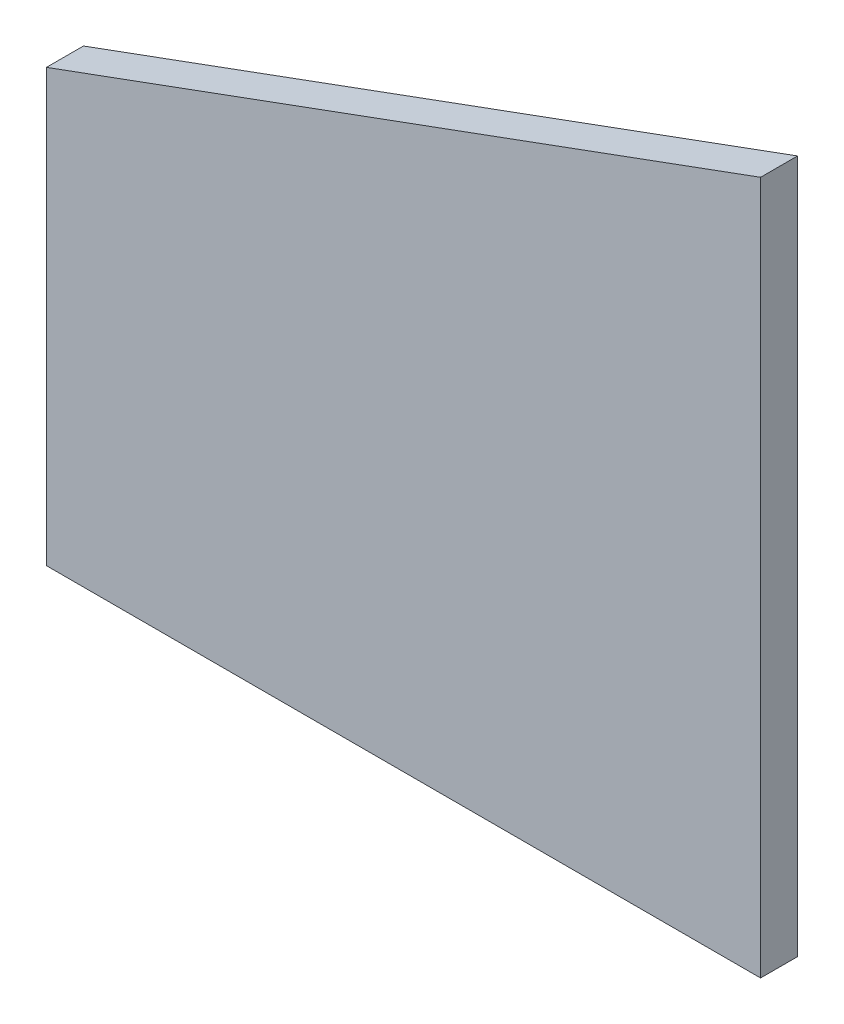
SolidWorks part; units mm, degrees
ref_plane "前视基准面" through (0, 0, 0) normal (0, 0, 1) x (1, 0, 0)
ref_plane "上视基准面" through (0, 0, 0) normal (0, 1, 0) x (1, 0, 0)
ref_plane "右视基准面" through (0, 0, 0) normal (1, 0, 0) x (0, 0, -1)
sketch "草图1" plane through (0, 0, 0) normal (0, 0, 1) x (1, 0, 0)
  line L2 (184.4778, 193) -> (184.4778, 286.3582)
  line L6 (184.4778, 286.3582) -> (338.9556, 343)
  line L7 (338.9556, 343) -> (338.9556, 193)
  line L8 (338.9556, 193) -> (184.4778, 193)
extrude "凸台-拉伸1" add sketch "草图1" along normal blind 8
